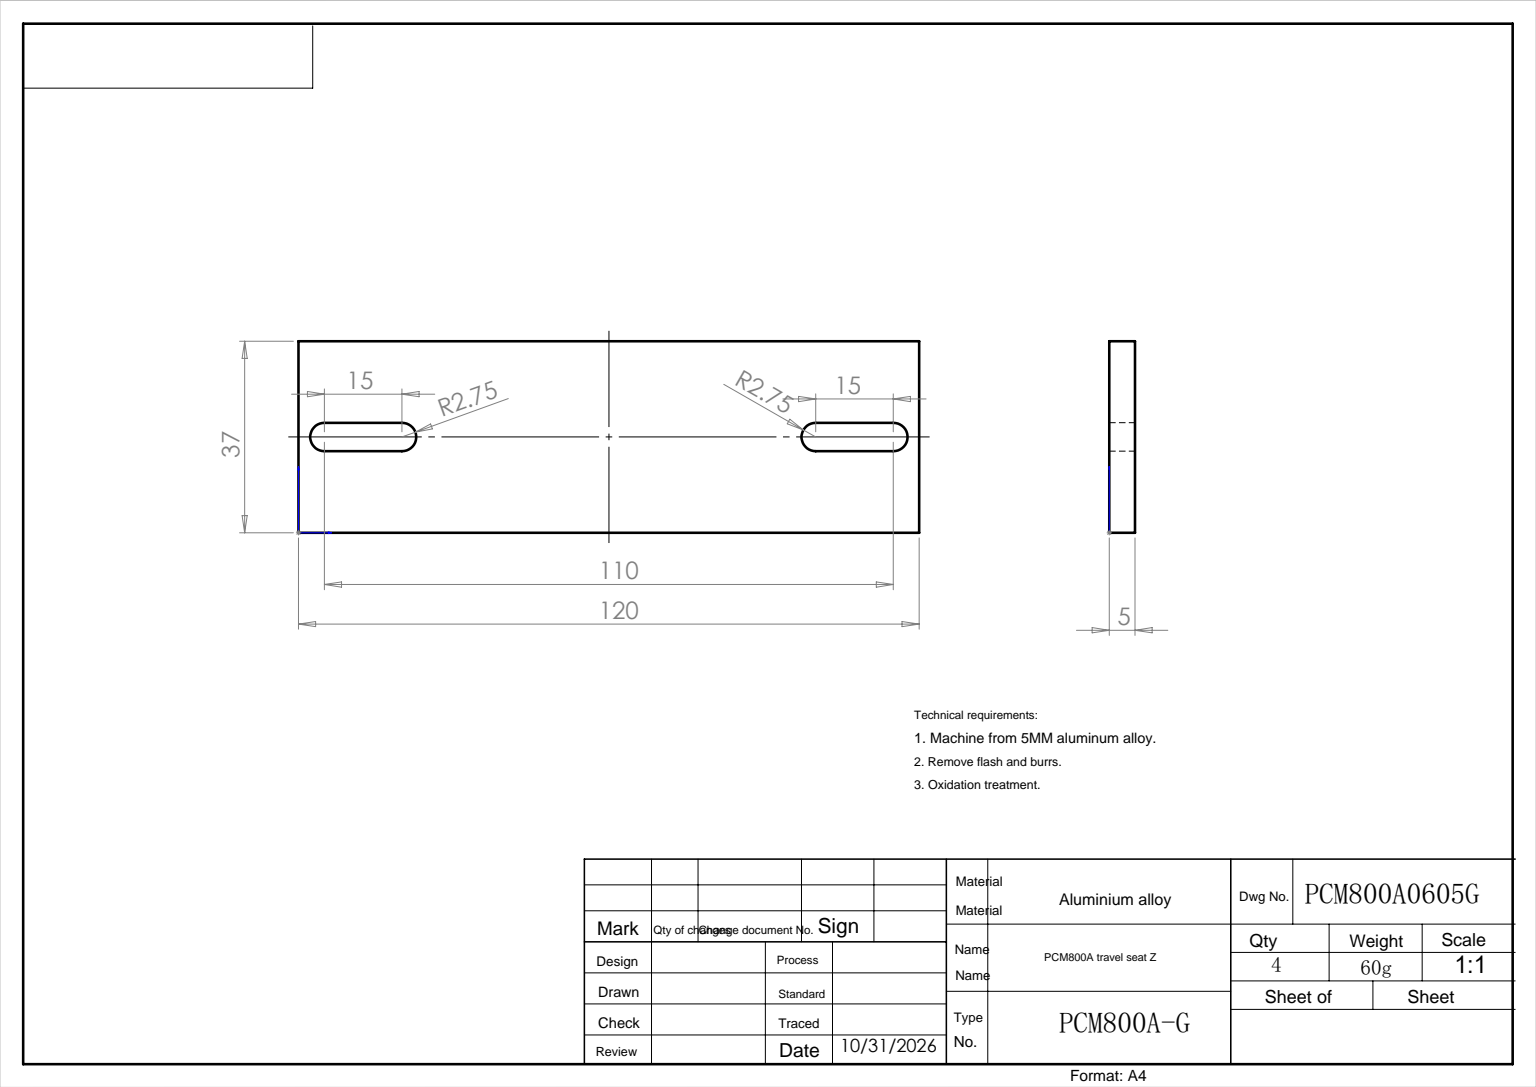
SolidWorks part; units mm, degrees
ref_plane "前视基准面" through (0, 0, 0) normal (0, 0, 1) x (1, 0, 0)
ref_plane "上视基准面" through (0, 0, 0) normal (0, 1, 0) x (1, 0, 0)
ref_plane "右视基准面" through (0, 0, 0) normal (1, 0, 0) x (0, 0, -1)
sketch "草图1" plane through (0, 0, 0) normal (0, 0, 1) x (1, 0, 0)
  line L0 (5, 21.25) -> (20, 21.25)
  line L1 (0, 0) -> (120, 0)
  line L2 (0, 0) -> (0, 37)
  line L3 (0, 37) -> (120, 37)
  line L4 (120, 0) -> (120, 37)
  line L5 (5, 15.75) -> (20, 15.75)
  line L6 (60, 37) -> (60, -11.4225) construction
  line L7 (115, 15.75) -> (100, 15.75)
  line L8 (115, 21.25) -> (100, 21.25)
  arc A0 (5, 21.25) -> (5, 15.75) centre (5, 18.5) ccw
  arc A1 (100, 15.75) -> (100, 21.25) centre (100, 18.5) cw
  arc A2 (20, 15.75) -> (20, 21.25) centre (20, 18.5) ccw
  arc A3 (115, 21.25) -> (115, 15.75) centre (115, 18.5) cw
  dimension "D3" = 5.5
  dimension "D5" = 18.5
  dimension "D7" = 5
  dimension "D9" = 15
  dimension "D10" = 5.5
  dimension "D14" = 18.5
  dimension "D1" = 120
  dimension "D2" = 37
extrude "凸台-拉伸1" add sketch "草图1" along normal blind 5
